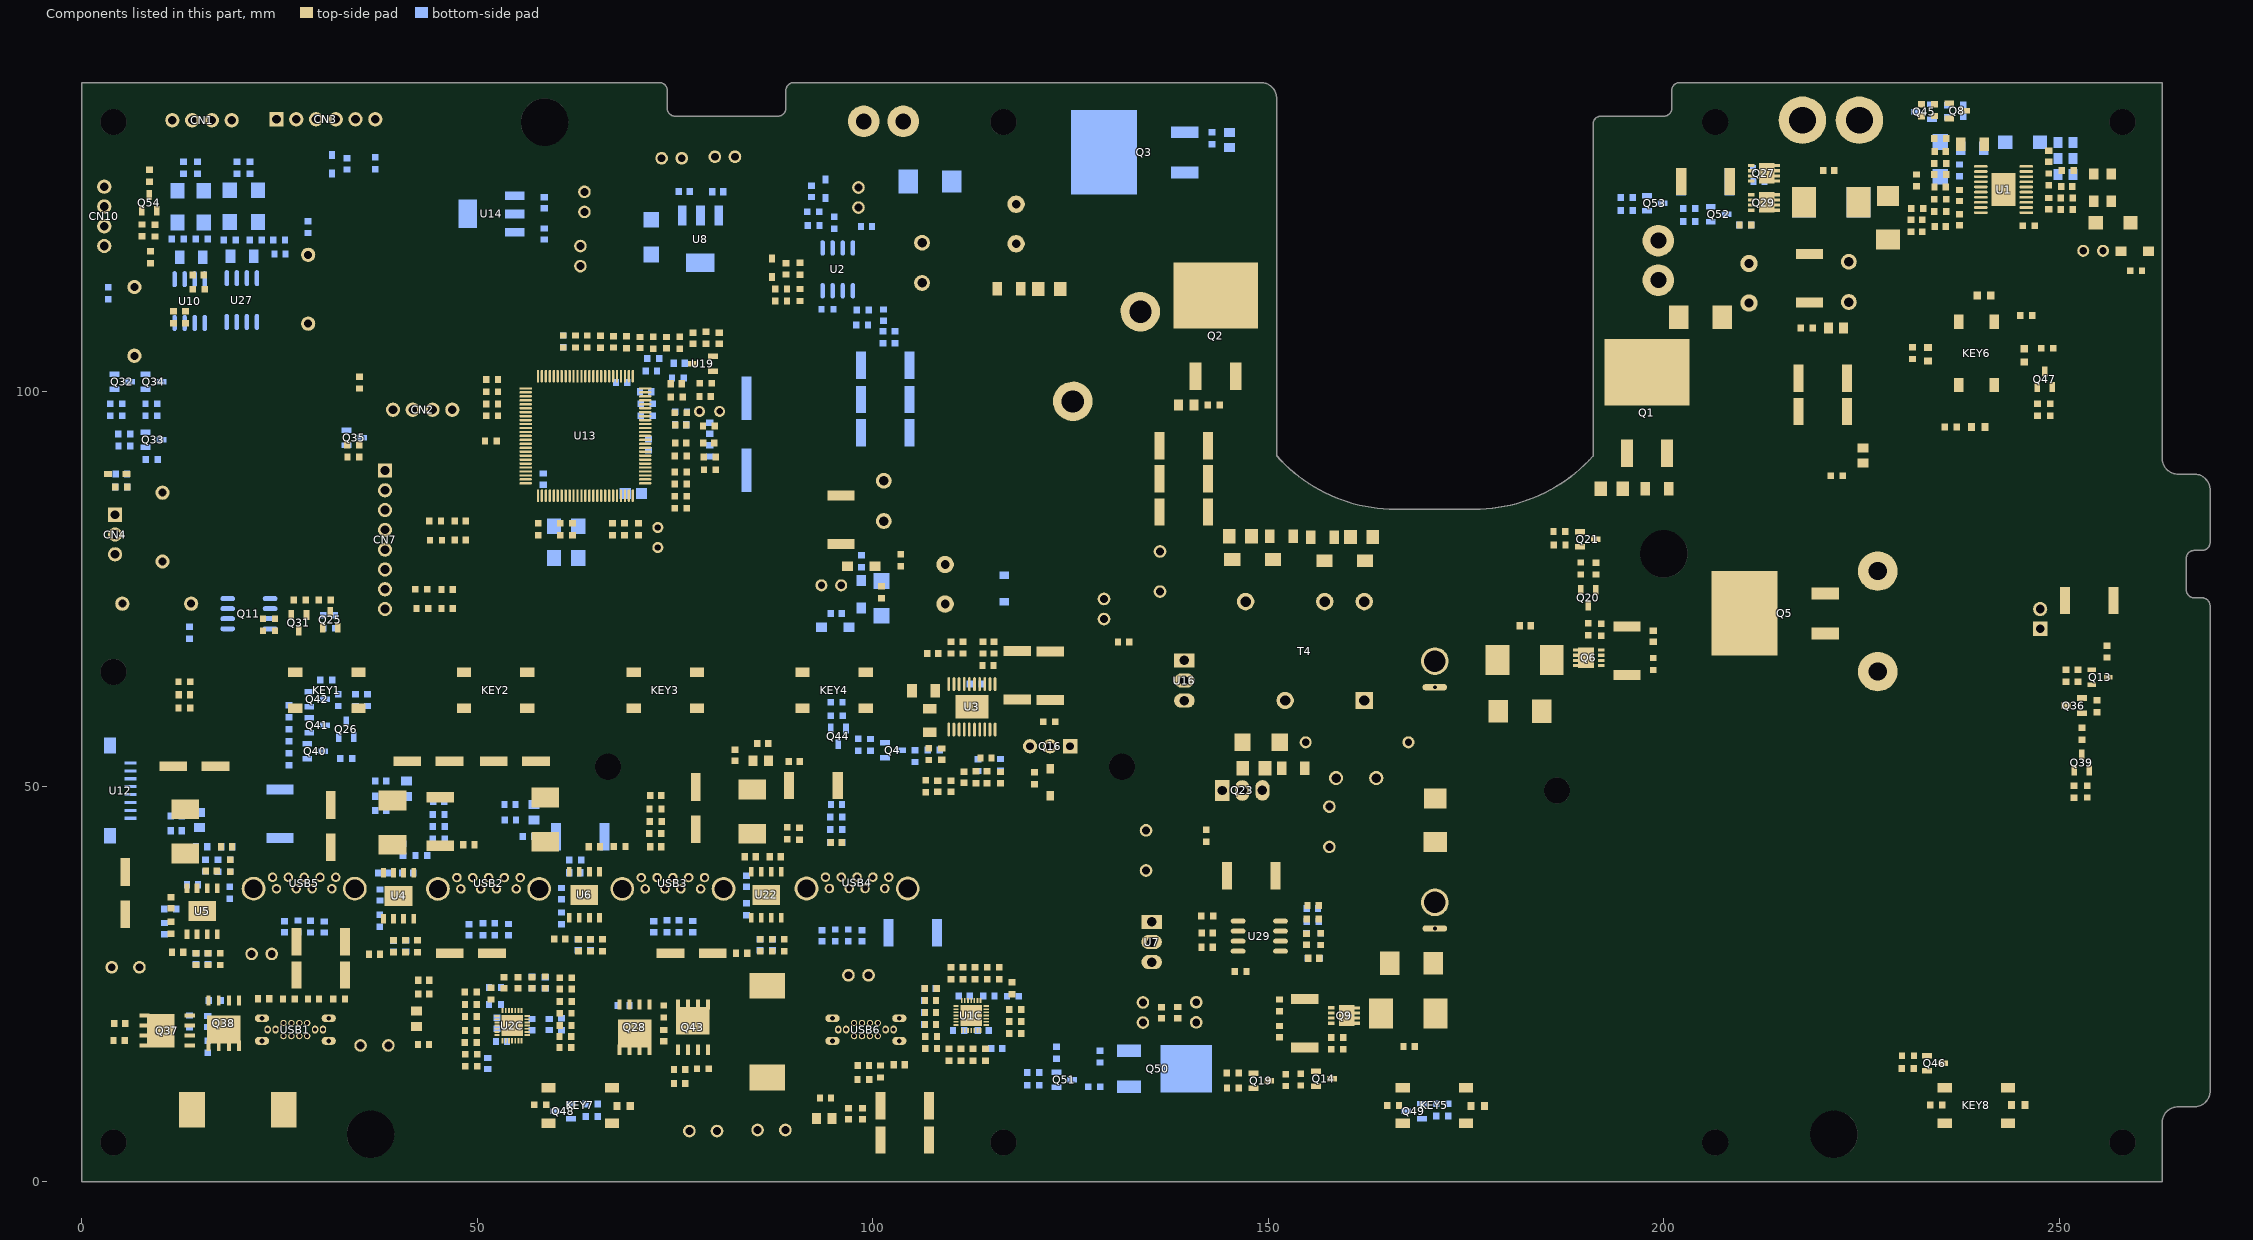
[diagram p0: the components of this part, seen from the top]
# Altium PCB MISC84402.PcbDoc (part 12 of 12)
Units mm, origin at the board's own origin, x right, y up, seen from the top; angles counter-clockwise.
Board outline 269.06 x 139 mm, 4 copper layers (TOP, GND02, PWR03, BOTTOM), stack 0.732 mm thick; 694 components, 428 nets, 1859 pads, 1384 vias.

## Other copper (continued)
PWR03:
  rectangle net B+: 115.189,120.904 121.666,126.238
  rectangle net B+: 207.772,110.566 212.852,112.09
  rectangle net B+: 209.525,108.763 211.226,111.049
  rectangle net GND: 193.802,117.653 199.212,120.193
  rectangle net GND: 194.996,118.897 197.764,121.818
  rectangle net BATA+: 102.616,131.445 105.156,136.906
  rectangle net BATA+: 104.267,132.461 106.934,135.382
  rectangle net GND: 97.409,131.191 100.711,137.033
  rectangle net GND: 95.758,132.969 98.552,135.255
  pour cut-out: 253.145,124.398 253.113,124.557 253.023,124.691 252.889,124.781 252.73,124.813 252.571,124.781 252.437,124.691 252.347,124.557 252.315,124.398 252.347,124.239 252.437,124.105 252.571,124.015 252.73,123.983 252.889,124.015 253.023,124.105 253.113,124.239
  pour cut-out: 191.515,49.5 191.472,50.154 191.344,50.798 191.133,51.419 190.843,52.007 190.479,52.553 190.046,53.046 189.553,53.478 189.008,53.843 188.419,54.133 187.798,54.344 187.155,54.472 186.5,54.515 185.845,54.472 185.202,54.344 184.581,54.133 183.992,53.843 183.447,53.478 182.954,53.046 182.521,52.553 182.157,52.007 181.867,51.419 181.656,50.798 181.528,50.154 181.485,49.5 181.528,48.845 181.656,48.202 181.867,47.581 182.157,46.992 182.521,46.447 182.954,45.954 183.447,45.521 183.992,45.157 184.581,44.866 185.202,44.656 185.845,44.528 186.5,44.485 187.155,44.528 187.798,44.656 188.419,44.866 189.008,45.157 189.553,45.521 190.046,45.954 190.479,46.447 190.843,46.992 191.133,47.581 191.344,48.202 191.472,48.845
  pour cut-out: 205.767,79.41 205.717,80.163 205.57,80.902 205.328,81.617 204.994,82.293 204.575,82.921 204.078,83.488 203.511,83.985 202.883,84.404 202.207,84.738 201.492,84.98 200.753,85.127 200,85.177 199.247,85.127 198.507,84.98 197.793,84.738 197.116,84.404 196.489,83.985 195.922,83.488 195.425,82.921 195.006,82.293 194.672,81.617 194.429,80.902 194.282,80.163 194.233,79.41 194.282,78.657 194.429,77.917 194.672,77.203 195.006,76.526 195.425,75.899 195.922,75.332 196.489,74.835 197.116,74.415 197.793,74.082 198.507,73.839 199.247,73.692 200,73.643 200.753,73.692 201.492,73.839 202.207,74.082 202.883,74.415 203.511,74.835 204.078,75.332 204.575,75.899 204.994,76.526 205.328,77.203 205.57,77.917 205.717,78.657
  pour cut-out: 226.515,6.03 226.472,6.685 226.344,7.328 226.133,7.949 225.843,8.538 225.479,9.083 225.046,9.576 224.553,10.009 224.008,10.373 223.419,10.663 222.798,10.874 222.155,11.002 221.5,11.045 220.845,11.002 220.202,10.874 219.581,10.663 218.992,10.373 218.447,10.009 217.954,9.576 217.521,9.083 217.157,8.538 216.866,7.949 216.656,7.328 216.528,6.685 216.485,6.03 216.528,5.375 216.656,4.732 216.866,4.111 217.157,3.522 217.521,2.977 217.954,2.484 218.447,2.051 218.992,1.687 219.581,1.396 220.202,1.186 220.845,1.058 221.5,1.015 222.155,1.058 222.798,1.186 223.419,1.396 224.008,1.687 224.553,2.051 225.046,2.484 225.479,2.977 225.843,3.522 226.133,4.111 226.344,4.732 226.472,5.375
  pour cut-out: 2.705,0.51 0.51,0.51 0.51,1.848 0.511,1.857 0.513,1.866 0.516,1.874 0.519,1.882 0.523,1.89 0.528,1.897 0.534,1.904 0.54,1.911 0.546,1.917 0.553,1.922 0.561,1.927 0.569,1.931 0.577,1.934 0.586,1.936 0.594,1.938 0.603,1.939 0.612,1.94 0.621,1.939 0.63,1.938 0.638,1.936 0.647,1.933 0.655,1.929 0.663,1.925 0.67,1.92 0.677,1.915 0.682,1.91 0.988,1.63 1.317,1.378 1.667,1.156 2.035,0.965 2.418,0.807 2.723,0.708 2.731,0.705 2.739,0.702 2.747,0.698 2.755,0.693 2.762,0.687 2.768,0.681 2.774,0.674 2.779,0.667 2.784,0.66 2.788,0.652 2.791,0.643 2.793,0.635 2.795,0.626 2.796,0.617 2.796,0.609 2.796,0.6 2.794,0.591 2.792,0.582 2.789,0.574 2.786,0.566 2.782,0.558 2.777,0.551 2.771,0.544 2.765,0.537 2.758,0.532 2.751,0.526 2.744,0.522 2.736,0.518 2.728,0.514 2.719,0.512 2.71,0.51
  pour cut-out: 262.49,136.598 262.489,136.589 262.487,136.58 262.484,136.572 262.481,136.564 262.477,136.556 262.472,136.549 262.466,136.542 262.46,136.535 262.454,136.529 262.447,136.524 262.439,136.519 262.431,136.515 262.423,136.512 262.414,136.51 262.406,136.508 262.397,136.507 262.388,136.506 262.379,136.507 262.37,136.508 262.362,136.51 262.353,136.513 262.345,136.517 262.337,136.521 262.33,136.526 262.323,136.531 262.317,136.537 262.311,136.544 262.305,136.551 262.302,136.556 262.063,136.922 261.793,137.265 261.494,137.583 261.168,137.874 260.819,138.135 260.556,138.302 260.549,138.307 260.542,138.312 260.535,138.318 260.529,138.325 260.524,138.332 260.519,138.34 260.515,138.348 260.512,138.356 260.51,138.364 260.508,138.373 260.507,138.382 260.506,138.391 260.507,138.399 260.508,138.408 260.51,138.417 260.513,138.425 260.516,138.433 260.521,138.441 260.526,138.449 260.531,138.456 260.537,138.462 260.544,138.468 260.551,138.473 260.558,138.478 260.566,138.482 260.574,138.485 260.583,138.488 260.592,138.49 260.598,138.49 262.49,138.49
  pour cut-out: 144.739,69.087 144.028,68.376 144.028,63.753 144.409,63.372 164.983,63.372 165.364,63.753 165.364,68.071 164.348,69.087
BOTTOM:
  rectangle net +13.6V-F: 109.347,92.075 126.238,97.536
  rectangle net +VCC_BAT: 97.155,117.196 98.933,120.015
  rectangle net GND: 200.431,117.551 200.939,119.452
  rectangle net GND: 209.423,114.554 211.201,117.856
  rectangle net GND: 208.407,115.57 212.217,117.15
  rectangle net GND: 222.631,114.554 224.155,117.983
  rectangle net GND: 221.615,115.57 225.425,116.967
  rectangle net +24V: 222.758,109.347 224.155,113.03
  rectangle net +24V: 221.742,110.617 225.044,112.014
  rectangle net +24V: 225.222,77.267 228.905,81.077
  rectangle net +24V: 221.539,74.32 230.607,78.994
  rectangle net NETC10_1: 196.748,86.233 208.686,94.996
  rectangle net B+: 209.753,108.585 211.785,111.125
  rectangle net B+: 207.899,110.363 213.106,112.268
  rectangle net +13.6V: 143.889,54.102 145.745,56.778
  rectangle net NETC170_2: 65.913,42.291 67.818,44.704
  rectangle net NETC170_2: 65.507,41.402 66.548,45.635
  rectangle net NETC33_1: 137.668,125.603 141.5,129.413
  rectangle net B+: 116.078,122.174 119.634,125.349
  rectangle net GND: 104.394,116.713 121.412,120.269
  rectangle net GND: 200.254,124.409 203.835,128.473
  rectangle net GND: 94.898,131.928 97.057,135.611
  rectangle net GND: 95.406,130.531 100.74,136.754
  rectangle net GND: 95.787,130.277 98.708,136.881
  rectangle net NETC40_2: 107.569,76.581 110.617,79.375
  rectangle net NETC192_2: 23.555,41.927 26.349,43.07
  rectangle net NETC192_2: 22.92,42.943 24.063,44.086
  rectangle net +13.6V: 142.339,54.178 144.196,56.854
  rectangle net +5V: 53.772,118.897 55.626,120.193
  rectangle net NETC41_1: 214.122,130.81 220.472,137.414
  rectangle net NETC41_2: 221.615,130.556 229.108,137.414
  rectangle net NETC41_2: 222.706,122.071 227.711,126.492
  rectangle net NETC41_1: 215.519,121.793 219.492,126.365
  rectangle net B+: 124.587,124.587 136.779,135.763
  rectangle net BATA+: 102.235,130.556 109.093,136.674
  rectangle net BATA+: 103.915,135.611 108.36,137.262
  rectangle net BATA+: 103.461,135.611 104.55,136.934
  rectangle net BATA+: 103.251,124.968 105.664,128.778
  rectangle net BATA+: 102.489,124.968 104.394,127.508
  rectangle net +13.6V-F: 104.648,112.268 108.331,114.935
  rectangle net +VCC_BAT: 97.155,119.634 97.917,121.793
  rectangle net +VCC_BAT: 97.155,121.412 98.933,124.079
  rectangle net +VCC_BAT: 98.298,119.761 98.933,121.793
  rectangle net +VCC_BAT: 97.536,120.523 98.425,121.031
  rectangle net +13.6V-F: 103.759,92.76 106.299,105.537
  rectangle net +13.6V-F: 120.65,94.234 125.222,101.143
  rectangle net BATA+: 102.489,125.456 105.986,129.286
  pour cut-out: 71.053,45.558 71.021,45.716 70.931,45.851 70.797,45.941 70.638,45.973 70.479,45.941 70.345,45.851 70.255,45.716 70.223,45.558 70.255,45.399 70.345,45.264 70.479,45.174 70.638,45.143 70.797,45.174 70.931,45.264 71.021,45.399
  pour cut-out: 6.014,73.117 5.983,73.352 5.892,73.571 5.748,73.759 5.56,73.903 5.341,73.994 5.106,74.025 4.871,73.994 4.652,73.903 4.464,73.759 4.319,73.571 4.229,73.352 4.198,73.117 4.229,72.882 4.319,72.663 4.464,72.475 4.652,72.33 4.871,72.239 5.106,72.208 5.341,72.239 5.56,72.33 5.748,72.475 5.892,72.663 5.983,72.882
  pour cut-out: 169.9,62.148 169.865,62.149 169.83,62.154 169.796,62.162 169.763,62.172 169.73,62.185 169.699,62.202 169.67,62.22 169.642,62.242 169.617,62.265 169.593,62.291 169.572,62.319 169.553,62.348 169.537,62.379 169.523,62.411 169.513,62.445 169.505,62.479 169.501,62.513 169.499,62.548 169.501,62.583 169.505,62.618 169.513,62.652 169.523,62.685 169.537,62.717 169.553,62.748 169.572,62.778 169.593,62.806 169.617,62.831 169.642,62.855 169.67,62.876 169.699,62.895 169.73,62.911 169.763,62.924 169.796,62.935 169.83,62.942 169.865,62.947 169.9,62.949 172.199,62.949 172.234,62.947 172.269,62.942 172.303,62.935 172.336,62.924 172.368,62.911 172.399,62.895 172.429,62.876 172.457,62.855 172.482,62.831 172.506,62.806 172.527,62.778 172.546,62.748 172.562,62.717 172.575,62.685 172.586,62.652 172.594,62.618 172.598,62.583 172.6,62.548 172.598,62.513 172.594,62.479 172.586,62.445 172.575,62.411 172.562,62.379 172.546,62.348 172.527,62.319 172.506,62.291 172.482,62.265 172.457,62.242 172.429,62.22 172.399,62.202 172.368,62.185 172.336,62.172 172.303,62.162 172.269,62.154 172.234,62.149 172.199,62.148
  pour cut-out: 169.899,31.648 169.864,31.65 169.83,31.654 169.795,31.662 169.762,31.672 169.73,31.686 169.699,31.702 169.669,31.721 169.642,31.742 169.616,31.765 169.592,31.791 169.571,31.819 169.552,31.848 169.536,31.879 169.523,31.912 169.512,31.945 169.505,31.979 169.5,32.014 169.499,32.048 169.5,32.083 169.505,32.118 169.512,32.152 169.523,32.185 169.536,32.218 169.552,32.249 169.571,32.278 169.592,32.306 169.616,32.332 169.642,32.355 169.669,32.376 169.699,32.395 169.73,32.411 169.762,32.425 169.795,32.435 169.83,32.443 169.864,32.447 169.899,32.449 172.199,32.449 172.234,32.447 172.269,32.443 172.303,32.435 172.336,32.425 172.368,32.411 172.399,32.395 172.429,32.376 172.457,32.355 172.482,32.332 172.506,32.306 172.527,32.278 172.546,32.249 172.562,32.218 172.575,32.185 172.586,32.152 172.594,32.118 172.598,32.083 172.6,32.048 172.598,32.014 172.594,31.979 172.586,31.945 172.575,31.912 172.562,31.879 172.546,31.848 172.527,31.819 172.506,31.791 172.482,31.765 172.457,31.742 172.429,31.721 172.399,31.702 172.368,31.686 172.336,31.672 172.303,31.662 172.269,31.654 172.234,31.65 172.199,31.648
  pour cut-out: 288 vertices and 0 holes, not listed, extent 5.957,25.834 11.075,28.794
  pour cut-out: 64.333,125.187 64.306,125.396 64.225,125.59 64.097,125.758 63.93,125.886 63.735,125.966 63.526,125.994 63.317,125.966 63.122,125.886 62.955,125.758 62.827,125.59 62.746,125.396 62.719,125.187 62.746,124.978 62.827,124.783 62.955,124.616 63.122,124.488 63.317,124.407 63.526,124.379 63.735,124.407 63.93,124.488 64.097,124.616 64.225,124.783 64.306,124.978
  pour cut-out: 144.473,70.929 143.838,70.294 143.838,64.198 144.219,63.817 164.793,63.817 165.174,64.198 165.174,70.421 164.666,70.929

## Silkscreen, mask and mechanical layers (free items; w line width, h text height)
Top Overlay:
  circle w0.152: c239.55,104.75 r15.45
  lines w0.127: 252.222,119.253 252.857,119.253 ; 252.357,125.857 252.857,125.857
  lines w0.152: 73.72,87.393 73.72,98.315 86.801,98.315 88.722,98.315 88.722,87.393 73.72,87.393 ; 230.632,21.45 249.55,21.45 249.55,71.45 230.632,71.45 230.632,21.45
  text "+" at 85.725,53.569 h1.02
  text "+" at 59.842,51.689 h1.02
  text "+" at 13.564,51.587 h1.02
  text "+" at 7.544,31.013 h1.02
Bottom Overlay:
  lines w0.152: 111.989,36.932 111.989,46.99 134.569,46.99 ; 112.014,36.932 134.671,36.932 ; 132.123,25.052 110.623,25.052 110.623,35.654 132.123,35.654 ; 136.289,58.097 114.789,58.097 114.789,68.699 136.289,68.699 ; 141.41,46.406 141.41,24.906 152.012,24.906 152.012,46.406 ; 158.445,49.962 181.102,49.962 ; 158.547,39.903 181.127,39.903 181.127,49.962
  text "+" at 110.744,128.803 h1.02
  text "+" at 67.437,121.742 h1.02
  text "+" at 60.452,118.999 h1.02
  text "+" at 117.881,114.986 h1.02
  text "+" at 132.664,113.64 h1.02
  text "+" at 48.616,80.594 h1.02
  text "+" at 68.148,75.997 h1.02
  text "+" at 60.706,75.946 h1.02
  text "+" at 115.367,75.54 h1.02
  text "+" at 53.772,75.387 h1.02
  text "+" at 139.573,71.247 h1.02
  text "+" at 132.283,69 h1.02
  text "+" at 134.29,25.502 h1.02
Top Solder:
  region: 101.092,138.43 101.092,134.845 100.966,134.826 100.928,134.953 100.718,135.345 100.437,135.688 100.094,135.97 99.702,136.179 99.277,136.308 99.216,136.314 99.216,134.086 99.216,131.859 99.277,131.865 99.702,131.994 100.094,132.203 100.437,132.485 100.718,132.828 100.928,133.22 100.966,133.347 101.092,133.329 101.092,131.191 102.362,129.921 102.743,129.54 105.918,129.54 106.299,129.159 106.299,121.793 107.188,120.904 110.109,120.904 110.617,120.396 110.617,116.84 110.49,116.713 103.632,116.713 101.727,118.618 100.584,119.761 100.584,123.825 100.584,127.508 99.695,128.397 99.441,128.651 93.345,128.651 92.583,129.413 92.583,138.557 92.702,138.676 100.846,138.676 hole: 98.454,136.314 98.393,136.308 97.968,136.179 97.577,135.97 97.234,135.688 96.952,135.345 96.743,134.953 96.614,134.528 96.608,134.468 98.454,134.468 hole: 98.454,133.706 96.608,133.706 96.614,133.645 96.743,133.22 96.952,132.828 97.234,132.485 97.577,132.203 97.968,131.994 98.393,131.865 98.454,131.859 hole: 106.593,119.945 106.593,119.127 107.412,119.127 107.307,119.378 107.106,119.64 106.844,119.841 hole: 105.831,119.945 105.58,119.841 105.318,119.64 105.117,119.378 105.013,119.127 105.831,119.127 hole: 107.412,118.365 106.593,118.365 106.593,117.546 106.844,117.651 107.106,117.852 107.307,118.114 hole: 105.831,118.365 105.013,118.365 105.117,118.114 105.318,117.852 105.58,117.651 105.831,117.546
  region: 109.017,123.673 110.007,122.682 122.809,122.682 123.901,123.774 123.901,124.79 124.435,125.324 134.595,125.324 135.509,126.238 135.509,134.036 134.188,135.357 123.723,135.357 122.453,134.087 122.453,130.378 120.421,128.346 109.677,128.346 109.017,127.686
  region: 120.117,84.963 121.844,83.236 132.08,83.236 133.96,85.115 133.96,101.498 140.233,107.772 148.285,107.772 148.768,108.255 148.768,132.004 147.193,133.579 139.7,133.579 138.811,132.69 138.811,124.104 137.566,122.86 130.175,122.86 127.279,119.964 127.279,104.343 129.54,102.083 129.54,95.555 127.533,93.548 121.895,93.548 120.117,91.77
OUTLINE:
  lines w0.025: 17.13,75.3 29.13,75.3 ; 17.13,105.3 29.13,105.3 ; 191.049,91.785 cw(c176.029,105.167) 176.029,85.05 166.081,85.05 cw(c166.081,105.12) 151.05,91.821 151.05,137 ccw(c149.05,137) 149.05,139 90,139 ccw(c90,138) 89,138 89,135.75 cw(c88,135.75) 88,134.75 75,134.75 cw(c75,135.75) 74,135.75 74,138 ccw(c73,138) 73,139 0,139 0,0 263,0 263,7.5 cw(c265,7.5) 265,9.5 267.058,9.5 ccw(c267.058,11.5) 269.058,11.5 269.058,72.85 ccw(c268.058,72.85) 268.058,73.85 267.058,73.85 cw(c267.058,74.85) 266.058,74.85 266.058,78.85 cw(c267.058,78.85) 267.058,79.85 268.058,79.85 ccw(c268.058,80.85) 269.058,80.85 269.058,87.5 ccw(c267.058,87.5) 267.058,89.5 265,89.5 cw(c265,91.5) 263,91.5 263,139 202,139 ccw(c202,138) 201,138 201,135.75 cw(c200,135.75) 200,134.75 192.05,134.75 ccw(c192.05,133.75) 191.05,133.75 191.05,91.785 ; 29.13,75.3 ccw(c29.13,77.3) 31.13,77.3 31.13,103.3 ccw(c29.13,103.3) 29.13,105.3 ; 29.13,75.3 15.13,75.3 cw(c15.13,77.3) 13.13,77.3 13.13,103.3 cw(c15.13,103.3) 15.13,105.3 29.13,105.3
DXF-0111-BOTTOM:
  drawing of 152 lines, arcs and shapes, not listed
DXF0111-TOP:
  drawing of 459 lines, arcs and shapes, not listed
  text "263.00" at 125.404,164.447 h1.02
  text "dia 6.00" at 169.394,91.376 h1.02
  text "139.00" at -38.85,68 h1.02
  text "dia 3.30" at 262.703,-3.472 h1.02
Mechanical 15:
  lines w1.016: -0.686,91.846 29.464,91.846 30.785,90.526 30.785,75.87 35.027,71.628 42.418,71.628 42.774,71.984 42.774,78.13 44.374,79.731 53.823,79.731 54.508,79.045 54.508,77.646 55.471,76.683 69.676,76.683 71.806,74.552 71.806,55.956 84.379,55.956 86.453,53.882 93.794,53.882 96.444,51.232 96.444,46.304 104.623,38.125 104.623,29.667 102.362,27.407 85.7,27.407 85.014,28.092 85.014,33.754 84.173,34.595 78.689,34.595 77.521,33.426 77.521,29.439 75.616,27.534 62.586,27.534 ; 29.167,32.69 22.081,25.603 14.351,25.603 13.487,26.467 13.487,31.902 9.271,36.119 9.271,53.086 11.227,55.042 18.948,55.042 22.962,51.029 34.214,51.029 38.927,55.742 71.843,55.742 ; 29.413,32.944 30.505,34.036 37.821,34.036 38.481,33.376 38.481,28.169 39.243,27.407 44.806,27.407 50.775,33.376 60.909,33.376 61.849,32.436 ; 58.973,23.9 56.926,21.853 56.219,21.853 55.88,21.514 55.88,18.567 54.782,17.469 54.782,16.16 55.855,15.088 65.761,15.088 67.094,16.421 67.094,22.898 ; 58.979,23.993 58.979,26.391 60.122,27.534 62.586,27.534 ; 61.849,29.718 61.849,28.27 62.586,27.534 ; 67.094,22.809 68.694,24.409 109.28,24.409 110.778,22.911 113.504,22.911 115.47,20.945 121.783,20.945 124.044,23.206 124.044,31.277 117.145,38.176 117.145,60.484 115.373,62.255 105.766,62.255 98.843,69.178 94.932,69.178 92.1,72.009 92.1,85.674 93.675,87.249 96.164,87.249 97.231,88.316 97.231,105.029 97.942,105.74 103.099,105.74 104.038,106.68 104.038,110.058 99.568,114.529 99.568,126.187 98.857,126.898 89.789,126.898 88.443,128.245 88.443,136.296 ; 61.849,32.436 61.849,29.261 61.849,32.436
Drill Drawing:
  text "CUTOUT" at 17.831,88.265 h1.02
  text ".Legend" at 277.292,49.2 h1.02

## Dimensions
0,0 to 269.058,11.5 on Drill Drawing
0,0 to 0,139 on Drill Drawing